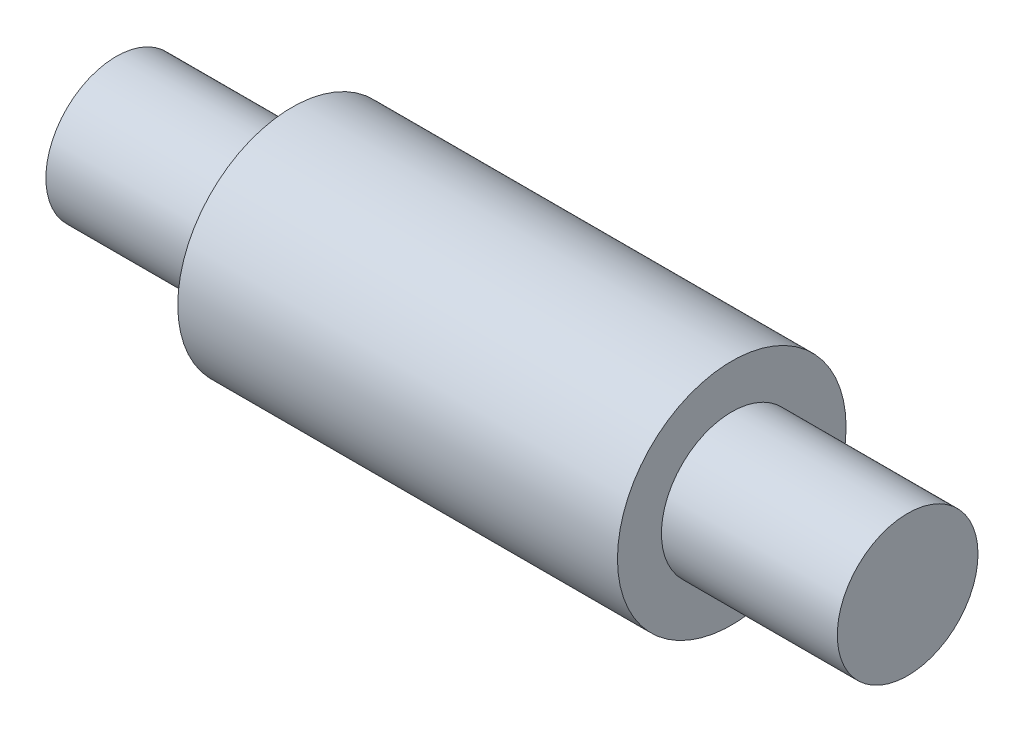
from build123d import *

# Parameters (mm, degrees)
SKETCH1_R           = 6.5
BOSS_EXTRUDE1_DEPTH = 12.5
SKETCH3_R           = 4
BOSS_EXTRUDE2_DEPTH = 10


with BuildPart() as part:
    # Sketch1 → Boss-Extrude1 (new, symmetric)
    with BuildSketch(Plane(origin=(0, 0, 0), x_dir=(0, 0, -1), z_dir=(1, 0, 0))):
        Circle(SKETCH1_R)
    extrude(amount=BOSS_EXTRUDE1_DEPTH, both=True)

    # Sketch3 → Boss-Extrude2 (add)
    with BuildSketch(Plane(origin=(12.5, 0, 0), x_dir=(0, 0, -1), z_dir=(1, 0, 0))):
        Circle(SKETCH3_R)
    boss_extrude2 = extrude(amount=BOSS_EXTRUDE2_DEPTH)

    # Mirror1: Boss-Extrude2 across plane
    add(boss_extrude2.mirror(Plane(origin=(0, 0, 0), x_dir=(0, 0, 1), z_dir=(1, 0, 0))))


solid = part.part
